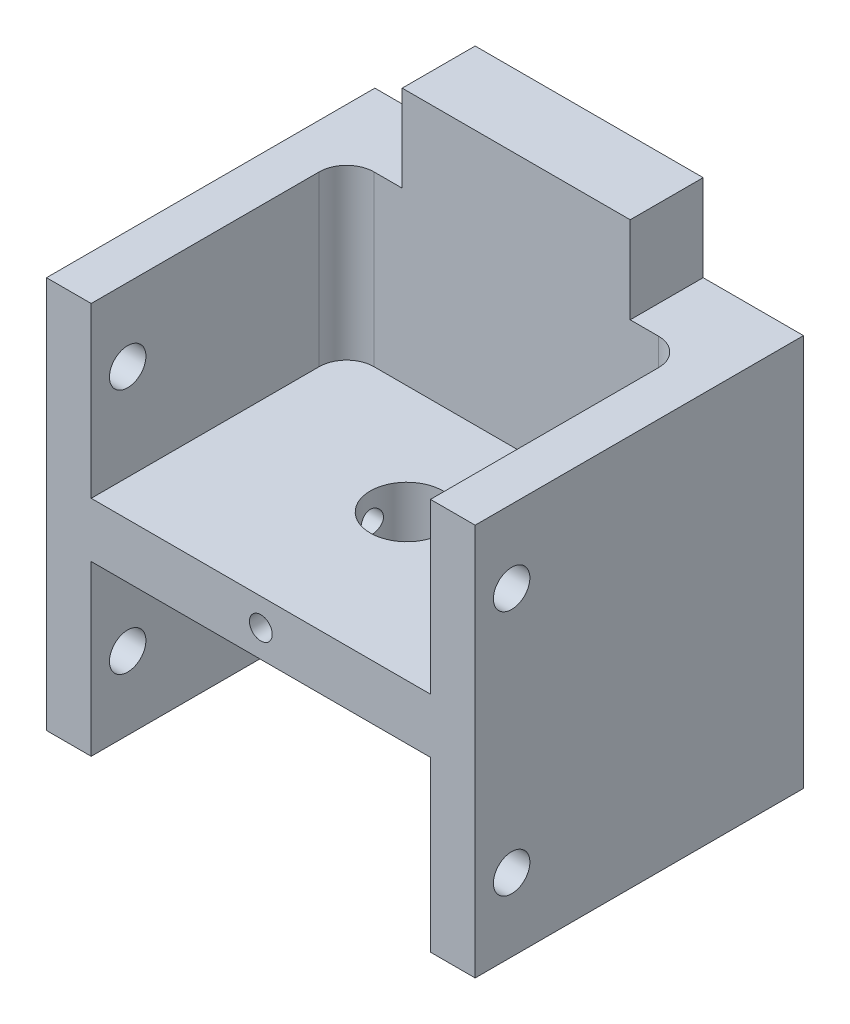
from build123d import *

# Parameters (mm, degrees)
SKETCH_1_W              = 47
SKETCH_1_H              = 43
EXTRUDE_1_DEPTH         = 36
SKETCH_2_W              = 37.2
SKETCH_2_H              = 43
CUT_EXTRUDE_1_DEPTH     = 28
CUT_EXTRUDE_2_REACH     = 64.986
SKETCH_3_R              = 2
SKETCH_4_W              = 37.2
SKETCH_4_H              = 6
EXTRUDE_2_DEPTH         = 28
FILLET_1_R              = 3
CUT_EXTRUDE_3_REACH     = 51.482
SKETCH_5_R              = 4
HOLE_WIZARD_M3_1_REACH  = 50.068
HOLE_WIZARD_M3_1_BORE_R = 1.25
HOLE_WIZARD_M3_2_REACH  = 57.419
HOLE_WIZARD_M3_2_BORE_R = 1.25
SKETCH_8_W              = 25
SKETCH_8_H              = 9.5
EXTRUDE_3_DEPTH         = 8
SKETCH_9_R              = 2.5
CUT_EXTRUDE_4_DEPTH     = 14


with BuildPart() as part:
    # 草图1 → 凸台-拉伸1 (new body)
    with BuildSketch(Plane.XY):
        Rectangle(SKETCH_1_W, SKETCH_1_H)
    extrude(amount=EXTRUDE_1_DEPTH)

    # 草图2 → 切除-拉伸1 (cut)
    with BuildSketch(Plane.XY.offset(36)):
        Rectangle(SKETCH_2_W, SKETCH_2_H)
    extrude(amount=-CUT_EXTRUDE_1_DEPTH, mode=Mode.SUBTRACT)

    # 切除-拉伸2: up to this face of the body (flat: up to its plane)
    cut_extrude_2_end = Plane(part.part.faces().sort_by_distance((23.5, 0, 18))[0])
    # 草图3 → 切除-拉伸2 (cut, up to the picked face)
    with BuildSketch(Plane.ZY.offset(23.5), mode=Mode.PRIVATE) as cut_extrude_2_sk1:
        with Locations((32, 13.5)):
            Circle(SKETCH_3_R)
    cut_extrude_2_tool1 = split(extrude(cut_extrude_2_sk1.sketch, amount=-CUT_EXTRUDE_2_REACH, mode=Mode.PRIVATE), bisect_by=cut_extrude_2_end, keep=Keep.BOTH, mode=Mode.PRIVATE)
    # 草图3 → 切除-拉伸2 (cut, up to the picked face)
    with BuildSketch(Plane.ZY.offset(23.5), mode=Mode.PRIVATE) as cut_extrude_2_sk2:
        with Locations((32, -13.5)):
            Circle(SKETCH_3_R)
    cut_extrude_2_tool2 = split(extrude(cut_extrude_2_sk2.sketch, amount=-CUT_EXTRUDE_2_REACH, mode=Mode.PRIVATE), bisect_by=cut_extrude_2_end, keep=Keep.BOTH, mode=Mode.PRIVATE)
    add(cut_extrude_2_tool1.solids().sort_by(Axis((-23.5, 13.5, 32), (1, 0, 0)))[0], mode=Mode.SUBTRACT)
    add(cut_extrude_2_tool2.solids().sort_by(Axis((-23.5, -13.5, 32), (1, 0, 0)))[0], mode=Mode.SUBTRACT)

    # 草图4 → 凸台-拉伸2 (add)
    with BuildSketch(Plane.XY.offset(8)):
        Rectangle(SKETCH_4_W, SKETCH_4_H)
    extrude(amount=EXTRUDE_2_DEPTH)

    # 圆角1
    fillet_1_edges = [part.edges().sort_by_distance(p)[0] for p in [
        (18.6, -12.25, 8),
        (-18.6, 12.25, 8),
        (18.6, 12.25, 8),
        (-18.6, -12.25, 8),
    ]]
    fillet(fillet_1_edges, radius=FILLET_1_R)

    # 草图5 → 切除-拉伸3 (cut, up to next)
    with BuildSketch(Plane(origin=(0, 3, 0), x_dir=(1, 0, 0), z_dir=(0, 1, 0)), mode=Mode.PRIVATE) as cut_extrude_3_sk1:
        with Locations(Location((0, -20, 0), (0, 0, 270))):
            Circle(SKETCH_5_R)
    cut_extrude_3_tool1 = extrude(cut_extrude_3_sk1.sketch, amount=-CUT_EXTRUDE_3_REACH, mode=Mode.PRIVATE) & part.part
    add(cut_extrude_3_tool1.solids().sort_by_distance((0, 3, 20))[0], mode=Mode.SUBTRACT)

    # M3 螺纹孔1 bore (on position points) → M3 螺纹孔1 (cut, up to next)
    with BuildSketch(Plane.XY.offset(36), mode=Mode.PRIVATE) as hole_wizard_m3_1_sk1:
        Circle(HOLE_WIZARD_M3_1_BORE_R)
    hole_wizard_m3_1_tool1 = extrude(hole_wizard_m3_1_sk1.sketch, amount=-HOLE_WIZARD_M3_1_REACH, mode=Mode.PRIVATE) & part.part
    add(hole_wizard_m3_1_tool1.solids().sort_by_distance((0, 0, 36))[0], mode=Mode.SUBTRACT)

    # M3 螺纹孔2 bore (on position points) → M3 螺纹孔2 (cut, up to next)
    with BuildSketch(Plane(origin=(-23.5, 0, 20), x_dir=(0, 0, -1), z_dir=(-1, 0, 0)), mode=Mode.PRIVATE) as hole_wizard_m3_2_sk1:
        Circle(HOLE_WIZARD_M3_2_BORE_R)
    hole_wizard_m3_2_tool1 = extrude(hole_wizard_m3_2_sk1.sketch, amount=-HOLE_WIZARD_M3_2_REACH, mode=Mode.PRIVATE) & part.part
    add(hole_wizard_m3_2_tool1.solids().sort_by_distance((-23.5, 0, 20))[0], mode=Mode.SUBTRACT)

    # 草图8 → 凸台-拉伸3 (add)
    with BuildSketch(Plane(origin=(0, 0, 0), x_dir=(-1, 0, 0), z_dir=(0, 0, -1))):
        with Locations((0, 26.25)):
            Rectangle(SKETCH_8_W, SKETCH_8_H)
        with Locations((0, -26.25)):
            Rectangle(SKETCH_8_W, SKETCH_8_H)
    extrude(amount=-EXTRUDE_3_DEPTH)

    # 草图9 → 切除-拉伸4 (cut)
    with BuildSketch(Plane.ZY.offset(23.5)):
        with Locations((20, 0)):
            Circle(SKETCH_9_R)
    extrude(amount=-CUT_EXTRUDE_4_DEPTH, mode=Mode.SUBTRACT)


solid = part.part
